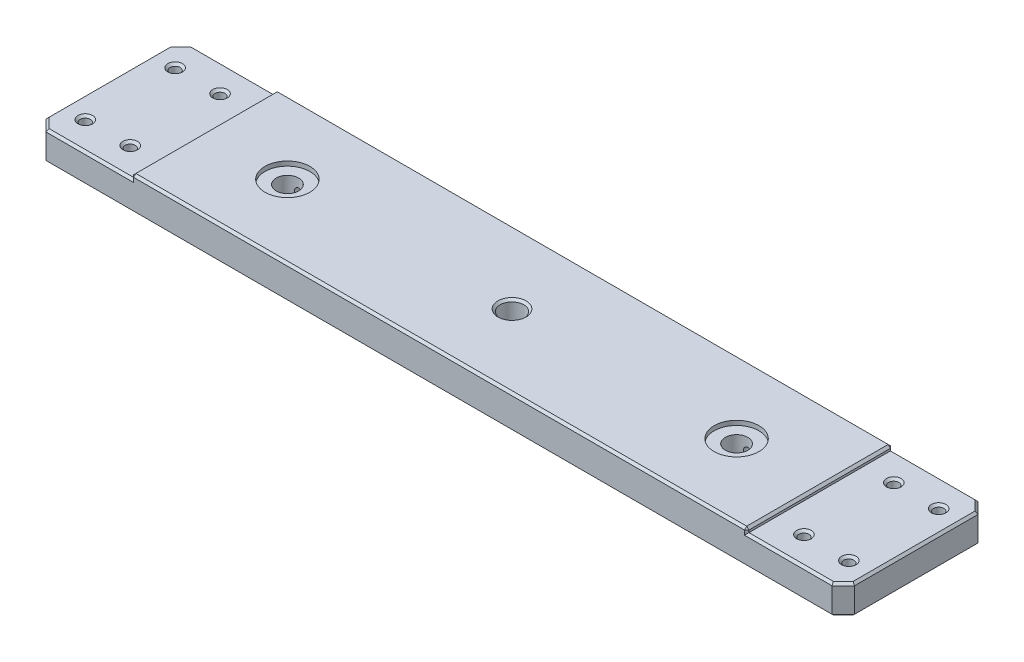
SolidWorks part; units mm, degrees
material "45"
ref_plane "Front Plane" through (0, 0, 0) normal (0, 0, 1) x (1, 0, 0)
ref_plane "Top Plane" through (0, 0, 0) normal (0, 1, 0) x (1, 0, 0)
ref_plane "Right Plane" through (0, 0, 0) normal (1, 0, 0) x (0, 0, -1)
sketch "Sketch1" plane through (0, 0, 0) normal (0, 1, 0) x (1, 0, 0)
  line L1 (-180, 32.5) -> (180, 32.5)
  line L2 (-180, 32.5) -> (-180, -32.5)
  line L3 (-180, -32.5) -> (180, -32.5)
  line L4 (180, 32.5) -> (180, -32.5)
  line L5 (-180, 32.5) -> (180, -32.5) construction
  line L6 (-180, -32.5) -> (180, 32.5) construction
  point P0 (0, 0)
  dimension "D1" = 65
  dimension "D2" = 360
extrude "Boss-Extrude1" add sketch "Sketch1" along normal blind 15
sketch "Sketch2" plane through (0, 15, 0) normal (0, 1, 0) x (1, 0, 0)
  line L0 (-180, -32.5) -> (180, -32.5) construction
  line L1 (-180, 32.5) -> (-137, 32.5)
  line L2 (-180, 32.5) -> (-180, -32.5)
  line L3 (-180, -32.5) -> (-137, -32.5)
  line L4 (-137, 32.5) -> (-137, -32.5)
  line L5 (0, 0) -> (0, -68.3379) construction
  line L6 (137, 32.5) -> (137, -32.5)
  line L7 (180, -32.5) -> (137, -32.5)
  line L8 (180, 32.5) -> (180, -32.5)
  line L9 (180, 32.5) -> (137, 32.5)
  dimension "D1" = 274
extrude "Cut-Extrude1" cut sketch "Sketch2" against normal blind 2
hole_wizard "Hole size (%based on) socket head cap screw type 1" positions "Sketch3" profile "Sketch4" counterbore size "M4" standard "GB" end condition through all
sketch "Sketch3" plane through (0, 0, 0) normal (0, -1, 0) x (-1, 0, 0)
  line L0 (170, -20) -> (170, 20)
  line L1 (170, 20) -> (150, 20)
  line L2 (150, 20) -> (150, -20)
  line L3 (150, -20) -> (170, -20)
  line L5 (0, 0) -> (0, 42.1688) construction
  line L7 (-150, -20) -> (-170, -20)
  line L8 (-150, 20) -> (-150, -20)
  line L9 (-170, 20) -> (-150, 20)
  line L10 (-170, -20) -> (-170, 20)
  point P0 (170, -20)
  point P2 (150, -20)
  point P4 (170, 20)
  point P6 (150, 20)
  point P24 (150, 0)
  point P25 (-150, 20)
  point P26 (-170, 20)
  point P27 (-150, -20)
  point P28 (-170, -20)
  dimension "D1" = 40
  dimension "D2" = 300
  dimension "D3" = 20
sketch "Sketch4" plane through (-170, 0, 20) normal (1, 0, 0) x (0, 0, -1)
  line L0 (0, 0) -> (0, 15)
  line L1 (0, 15) -> (2.25, 15)
  line L3 (2.25, 15) -> (2.25, 4.6)
  line L4 (2.25, 4.6) -> (4, 4.6)
  line L5 (4, 4.6) -> (4, 0)
  line L7 (4, 0) -> (0, 0)
  line L11 (0, -6.35) -> (0, 107.95) construction
  dimension "通孔孔直径" = 4.5
  dimension "通孔孔深度" = 15
  dimension "柱形沉头孔直径" = 8
  dimension "柱形沉头孔深度" = 4.6
hole_wizard "M12x1.5 Tapped Hole1" positions "Sketch5" profile "Sketch6" tap size "M12x1.5" standard "GB" end condition through all
sketch "Sketch5" plane through (0, 0, 0) normal (0, -1, 0) x (-1, 0, 0)
  point P0 (0, 0)
sketch "Sketch6" plane through (0, 0, 0) normal (1, 0, 0) x (0, 0, -1)
  line L0 (0, 0) -> (0, 15)
  line L1 (0, 15) -> (5.25, 15)
  line L2 (5.25, 15) -> (5.25, 0)
  line L5 (5.25, 0) -> (0, 0)
  line L11 (0, -6.35) -> (0, 107.95) construction
  dimension "通孔螺纹孔钻头直径" = 10.5
  dimension "通孔螺纹孔钻头深度" = 15
cosmetic thread "Hole Thread1" parameters "D2"=12
chamfer "Chamfer1" distance 5 angle 45 4 edges at (-180, 6.5, 32.5) (-180, 6.5, -32.5) (180, 6.5, 32.5) (180, 6.5, -32.5)
chamfer "Chamfer2" distance 1 angle 45 44 edges at (177.5, 0, 30) (180, 0, 0) (177.5, 0, -30) (0, 0, -32.5) (-177.5, 0, -30) (-180, 0, 0) (-177.5, 0, 30) (0, 0, 32.5) (170, 0, 16) (150, 0, 16) (170, 0, -24) (150, 0, -24) (-150, 0, -24) (-170, 0, -24) (-150, 0, 16) (-170, 0, 16) (0, 0, -5.25) (0, 15, -5.25) (170, 13, 22.25) (150, 13, 22.25) (150, 13, -17.75) (170, 13, -17.75) (-170, 13, -17.75) (-150, 13, -17.75) (-150, 13, 22.25) (-170, 13, 22.25) (137, 14, 32.5) (156, 13, 32.5) (177.5, 13, 30) (180, 13, 0) (177.5, 13, -30) (156, 13, -32.5) (137, 15, 0) (137, 14, -32.5) (0, 15, -32.5) (0, 15, 32.5) (-137, 14, 32.5) (-137, 15, 0) (-137, 14, -32.5) (-156, 13, -32.5) (-177.5, 13, -30) (-180, 13, 0) (-177.5, 13, 30) (-156, 13, 32.5)
sketch "Sketch7" plane through (0, 15, 0) normal (0, 1, 0) x (1, 0, 0)
  line L0 (0, 0) -> (0, 72.858) construction
  circle A0 centre (-100, 0) radius 5
  circle A1 centre (100, 0) radius 5
  dimension "D1" = 200
  dimension "D2" = 10
extrude "Cut-Extrude2" cut sketch "Sketch7" against normal through all
hole_wizard "M4 Tapped Hole1" positions "Sketch8" profile "Sketch9" tap size "M4" standard "GB"
sketch "Sketch8" plane through (0, 0, -32.5) normal (0, 0, -1) x (-1, 0, 0)
  line L0 (0, 0) -> (0, 31.2975) construction
  point P0 (-100, 7.5)
  point P9 (100, 7.5)
  dimension "D1" = 7.5
  dimension "D2" = 100
sketch "Sketch9" plane through (100, 7.5, -32.5) normal (1, 0, 0) x (0, 1, 0)
  line L0 (0, 0) -> (0, 27.5)
  line L1 (0, 27.5) -> (1.65, 27.5)
  line L2 (1.65, 27.5) -> (1.65, 0)
  line L5 (1.65, 0) -> (0, 0)
  line L11 (0, -6.35) -> (0, 107.95) construction
  dimension "通孔螺纹孔钻头直径" = 3.3
  dimension "通孔螺纹孔钻头深度" = 27.5
cosmetic thread "Hole Thread2" parameters "D2"=4
cosmetic thread "Hole Thread3" parameters "D2"=4
sketch "Sketch10" plane through (0, 15, 0) normal (0, 1, 0) x (1, 0, 0)
  circle A0 centre (-100, 0) radius 10
  circle A1 centre (100, 0) radius 10
  dimension "D1" = 20
extrude "Cut-Extrude3" cut sketch "Sketch10" against normal blind 2
